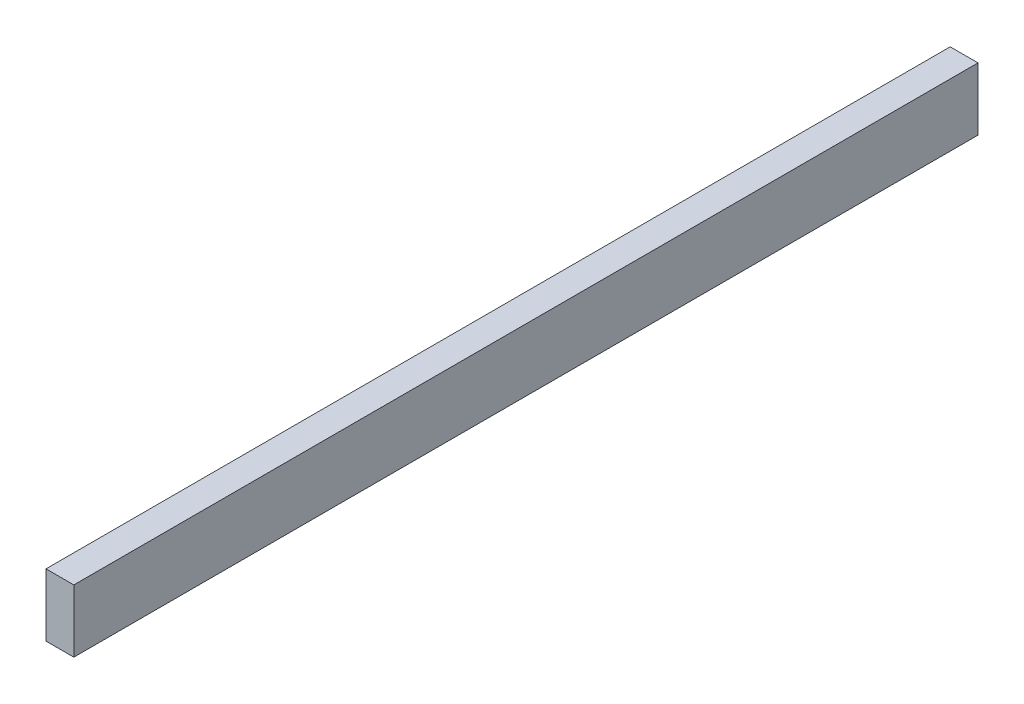
SolidWorks part; units mm, degrees
ref_plane "前视基准面" through (0, 0, 0) normal (0, 0, 1) x (1, 0, 0)
ref_plane "上视基准面" through (0, 0, 0) normal (0, 1, 0) x (1, 0, 0)
ref_plane "右视基准面" through (0, 0, 0) normal (1, 0, 0) x (0, 0, -1)
other "Configuration Table"
sketch "草图1" plane through (0, 0, 0) normal (0, 0, 1) x (1, 0, 0)
  line L0 (-4, -9) -> (4, -9)
  line L1 (4, -9) -> (4, 9)
  line L2 (4, 9) -> (-4, 9)
  line L3 (-4, 9) -> (-4, -9)
  point P0 (0, 0)
  dimension "D1" = 4
  dimension "D2" = 8
  dimension "D3" = 9
  dimension "D4" = 18
extrude "凸台-拉伸1" add sketch "草图1" against normal mid plane 260
